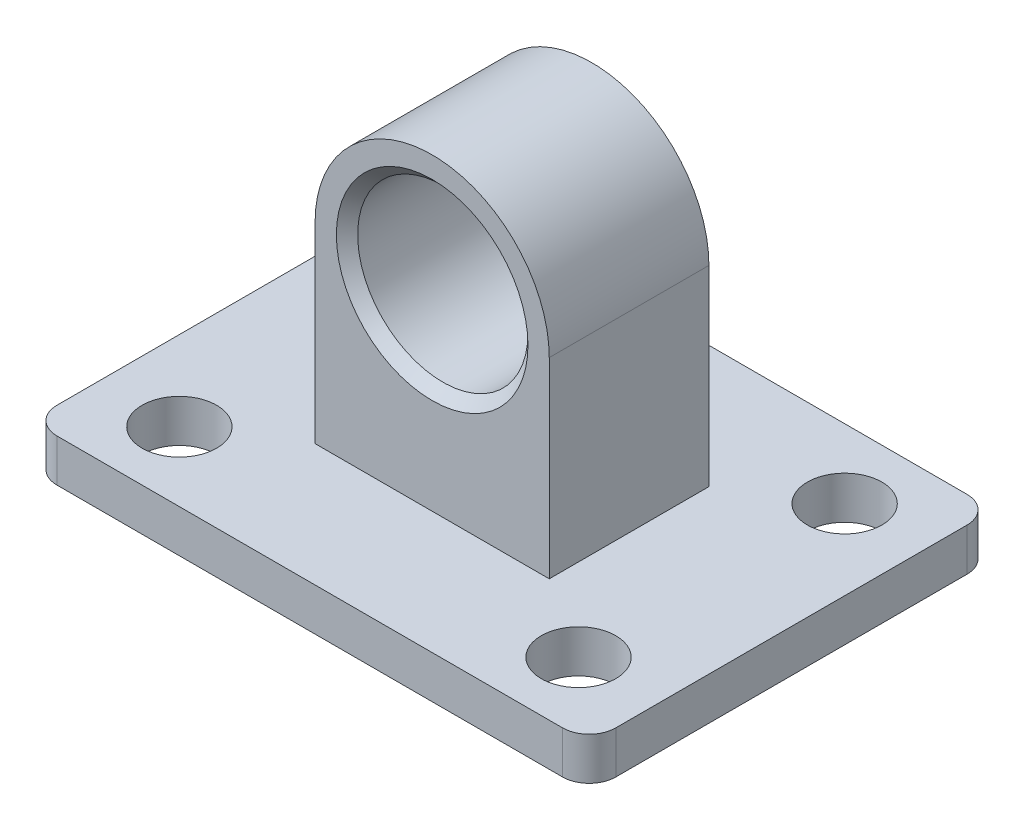
from build123d import *

# Parameters (mm, degrees)
SKETCH_1_R      = 7
EXTRUDE_1_DEPTH = 8
SKETCH_2_R      = 16
EXTRUDE_2_DEPTH = 15
CHAMFER_1_SIZE  = 2


with BuildPart() as part:
    # 草图1 → 凸台-拉伸1 (new body)
    with BuildSketch(Plane(origin=(0, 0, 0), x_dir=(1, 0, 0), z_dir=(0, 1, 0))):
        with BuildLine():
            Line((-47.5, -38), (47.5, -38))
            ThreePointArc((47.5, -38), (51.035533906, -36.535533906), (52.5, -33))
            Line((52.5, -33), (52.5, 33))
            ThreePointArc((52.5, 33), (51.035533906, 36.535533906), (47.5, 38))
            Line((47.5, 38), (-47.5, 38))
            ThreePointArc((-47.5, 38), (-51.035533906, 36.535533906), (-52.5, 33))
            Line((-52.5, 33), (-52.5, -33))
            ThreePointArc((-52.5, -33), (-51.035533906, -36.535533906), (-47.5, -38))
        make_face()
        with Locations(Location((-37.5, -25, 0), (0, 0, 270))):
            Circle(SKETCH_1_R, mode=Mode.SUBTRACT)
        with Locations(Location((37.5, -25, 0), (0, 0, 90))):
            Circle(SKETCH_1_R, mode=Mode.SUBTRACT)
        with Locations(Location((-37.5, 25, 0), (0, 0, 90))):
            Circle(SKETCH_1_R, mode=Mode.SUBTRACT)
        with Locations(Location((37.5, 25, 0), (0, 0, 270))):
            Circle(SKETCH_1_R, mode=Mode.SUBTRACT)
    extrude(amount=EXTRUDE_1_DEPTH)


with BuildPart() as body_2:
    # 草图2 → 凸台-拉伸2 (new, symmetric)
    with BuildSketch(Plane.XY):
        with BuildLine():
            Line((-22, 44), (-22, 8))
            Line((-22, 8), (22, 8))
            Line((22, 8), (22, 44))
            ThreePointArc((22, 44), (0, 66), (-22, 44))
        make_face()
        with Locations((0, 44)):
            Circle(SKETCH_2_R, mode=Mode.SUBTRACT)
    extrude(amount=EXTRUDE_2_DEPTH, both=True)

    # 倒角1
    chamfer_1_edges = [body_2.edges().sort_by_distance(p)[0] for p in [
        (-16, 44, -15),
        (-16, 44, 15),
    ]]
    chamfer(chamfer_1_edges, length=CHAMFER_1_SIZE)


solid = Compound([part.part, body_2.part])
